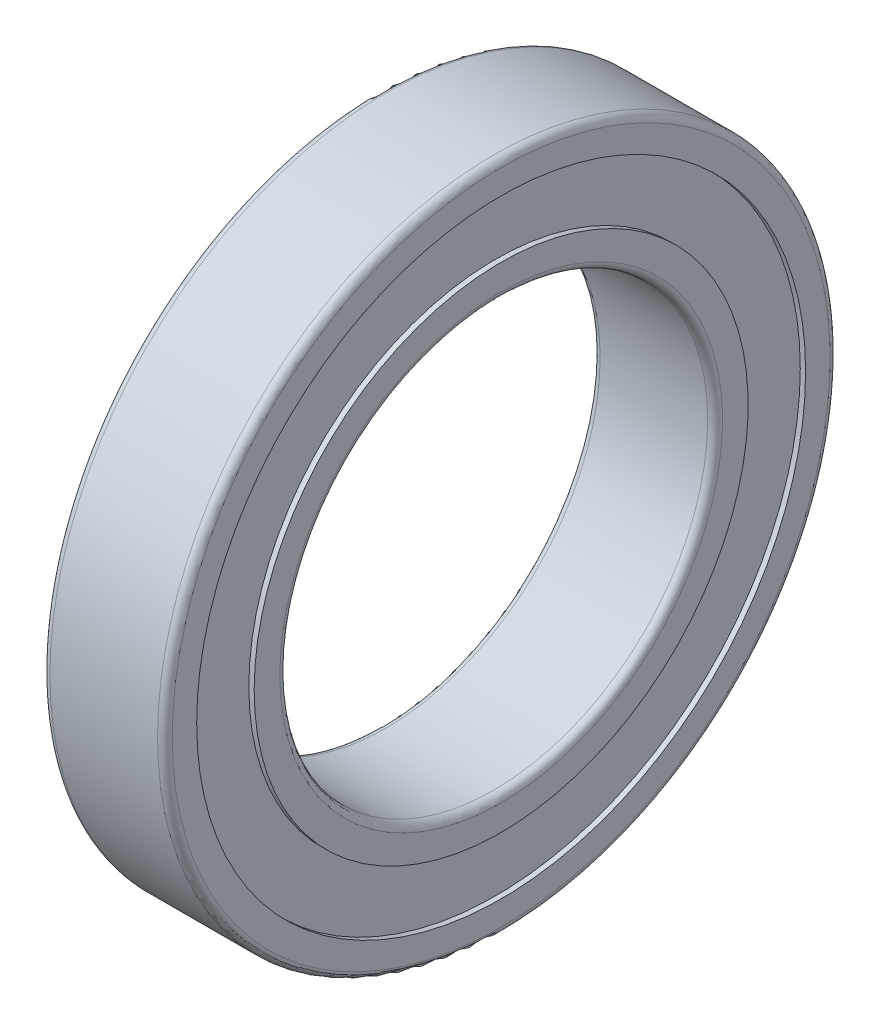
from build123d import *

# Parameters (mm, degrees)
FILLET1_R = 0.6
FILLET2_R = 0.6


with BuildPart() as part:
    # Sketch1 → Revolve1 (revolve)
    with BuildSketch(Plane.XY, mode=Mode.PRIVATE) as revolve1_sk:
        Polygon((0, 17.5), (10, 17.5), (10, 20.2), (9.565, 20.2), (9.565, 24.9), (10, 24.9), (10, 27.5), (0, 27.5), (0, 24.9), (0.435, 24.9), (0.435, 20.2), (0, 20.2), align=None)
    revolve(revolve1_sk.sketch.rotate(Axis((0, 0, 0), (1, 0, 0)), 90), axis=Axis((0, 0, 0), (1, 0, 0)))

    # Fillet1
    fillet1_edges = [part.edges().sort_by_distance(p)[0] for p in [
        (0, 0, -27.5),
        (10, 0, -27.5),
    ]]
    fillet(fillet1_edges, radius=FILLET1_R)

    # Fillet2
    fillet2_edges = [part.edges().sort_by_distance(p)[0] for p in [
        (10, 0, -17.5),
        (0, 0, -17.5),
    ]]
    fillet(fillet2_edges, radius=FILLET2_R)


solid = part.part
